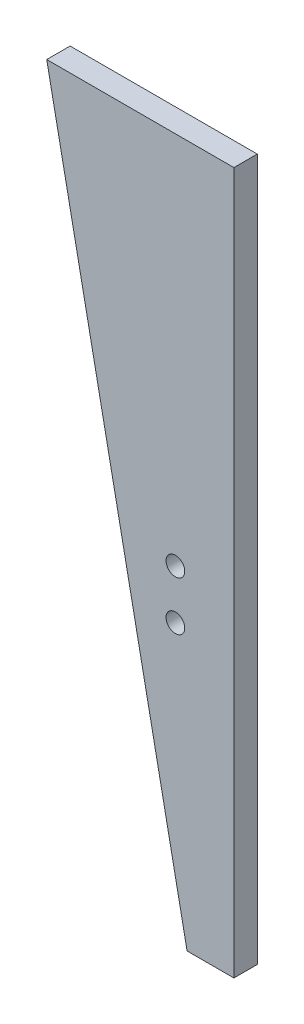
from build123d import *

# Parameters (mm, degrees)
EXTRUDE1_DEPTH = 5
SKETCH2_R      = 4
EXTRUDE2_DEPTH = 10


with BuildPart() as part:
    # Sketch1 → Extrude1 (new, symmetric)
    with BuildSketch(Plane.XY):
        Polygon((-80, 0), (0, 0), (0, -300), (-20, -300), align=None)
    extrude(amount=EXTRUDE1_DEPTH, both=True)

    # Sketch2 → Extrude2 (cut)
    with BuildSketch(Plane.XY.offset(5)):
        with Locations((-25, -160)):
            Circle(SKETCH2_R)
        with Locations((-25, -181)):
            Circle(SKETCH2_R)
    extrude(amount=-EXTRUDE2_DEPTH, mode=Mode.SUBTRACT)


solid = part.part
